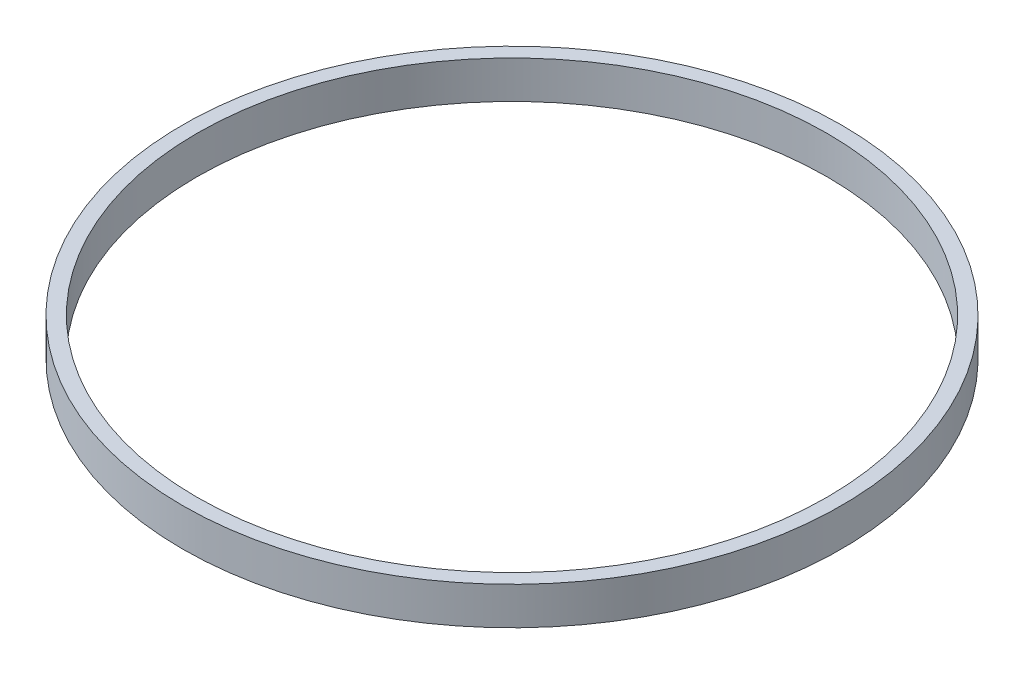
from build123d import *

# Parameters (mm, degrees)
SKETCH1_R           = 26.25
SKETCH1_R_2         = 25.1
BOSS_EXTRUDE1_DEPTH = 3


with BuildPart() as part:
    # Sketch1 → Boss-Extrude1 (new body)
    with BuildSketch(Plane(origin=(0, 0, 0), x_dir=(1, 0, 0), z_dir=(0, 1, 0))):
        with Locations(Location((0, 0, 0), (0, 0, 270))):
            Circle(SKETCH1_R)
        with Locations(Location((0, 0, 0), (0, 0, 270))):
            Circle(SKETCH1_R_2, mode=Mode.SUBTRACT)
    extrude(amount=BOSS_EXTRUDE1_DEPTH)


solid = part.part
